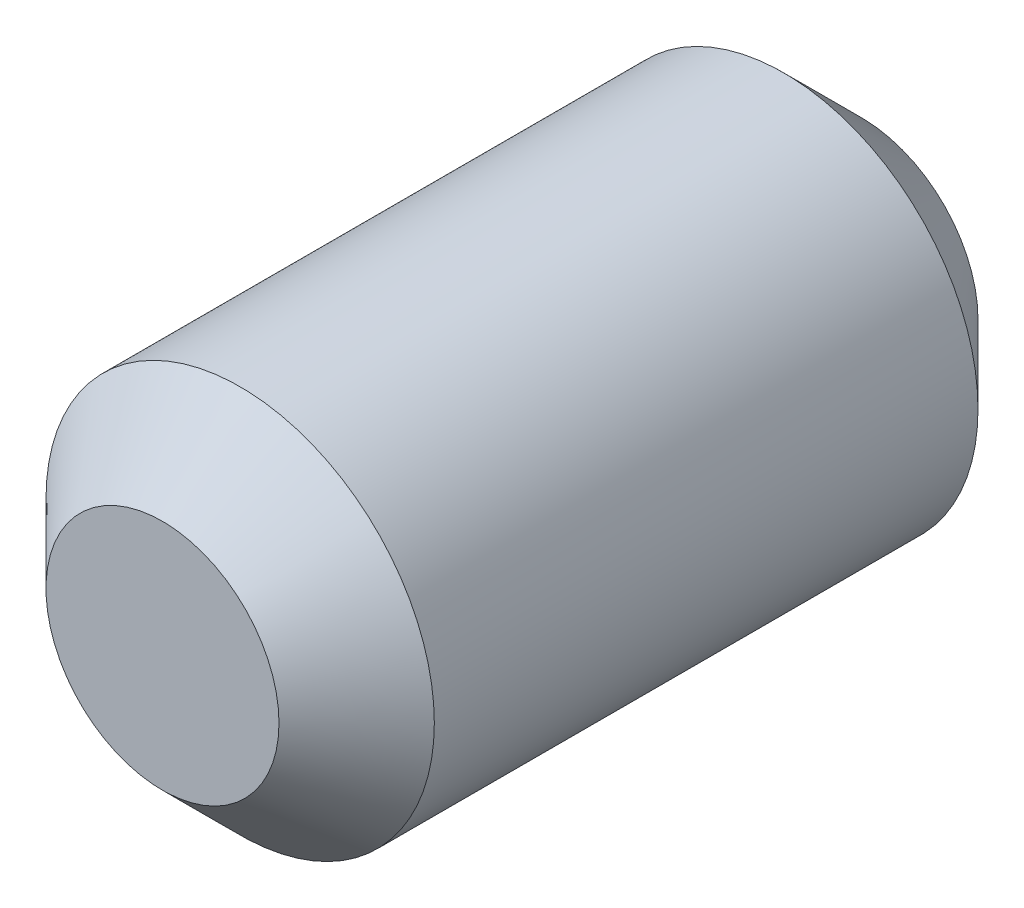
SolidWorks part; units mm, degrees
ref_plane "Front Plane" through (0, 0, 0) normal (0, 0, 1) x (1, 0, 0)
ref_plane "Top Plane" through (0, 0, 0) normal (0, 1, 0) x (1, 0, 0)
ref_plane "Right Plane" through (0, 0, 0) normal (1, 0, 0) x (0, 0, -1)
sketch "Sketch1" plane through (0, 0, 0) normal (0, 0, 1) x (1, 0, 0)
  circle A0 centre (0, 0) radius 2.5
  dimension "D1" = 5
extrude "Boss-Extrude1" add sketch "Sketch1" along normal blind 9
chamfer "Chamfer1" distance 1 angle 45 2 edges at (2.5, 0, 0) (2.5, 0, 9)
